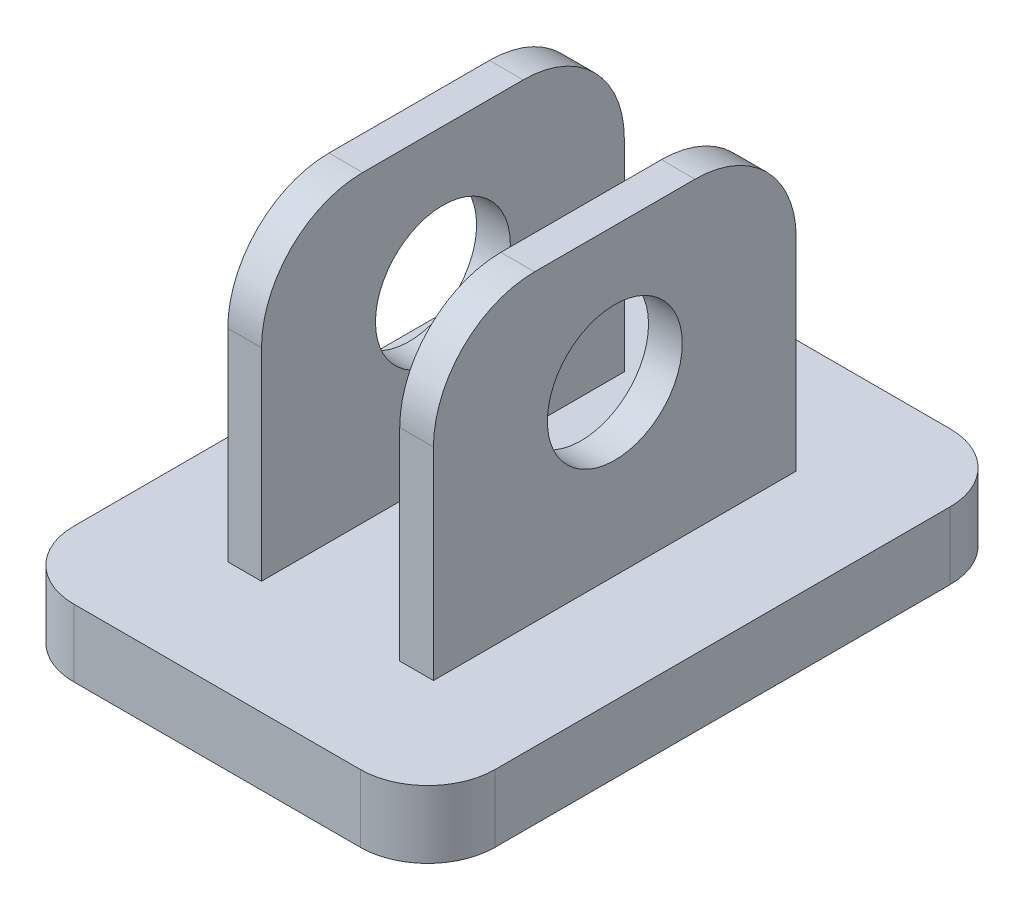
SolidWorks part; units mm, degrees
other "Objet de détail1"
other "Objet de détail2"
other "Dossier de soudure"
other "Cordon de soudure1"
other "Cordon de soudure2"
ref_plane "Plan de face" through (0, 0, 0) normal (0, 0, 1) x (1, 0, 0)
ref_plane "Plan de dessus" through (0, 0, 0) normal (0, 1, 0) x (1, 0, 0)
ref_plane "Plan de droite" through (0, 0, 0) normal (1, 0, 0) x (0, 0, -1)
sketch "Sketch1" plane through (0, 0, 0) normal (0, 1, 0) x (1, 0, 0)
  line L1 (-8.5, -17.5) -> (8.5, -17.5)
  line L2 (-12.5, -13.5) -> (-12.5, 13.5)
  line L3 (-8.5, 17.5) -> (8.5, 17.5)
  line L4 (12.5, -13.5) -> (12.5, 13.5)
  line L5 (0, 17.5) -> (0, -17.5) construction
  line L6 (-12.5, 0) -> (12.5, 0) construction
  arc A0 (8.5, -17.5) -> (12.5, -13.5) centre (8.5, -13.5) ccw
  arc A1 (-8.5, -17.5) -> (-12.5, -13.5) centre (-8.5, -13.5) cw
  arc A2 (8.5, 17.5) -> (12.5, 13.5) centre (8.5, 13.5) cw
  arc A3 (-12.5, 13.5) -> (-8.5, 17.5) centre (-8.5, 13.5) cw
  point P0 (0, 0)
  point P9 (-12.5, -17.5)
  point P12 (12.5, 17.5)
  point P15 (-12.5, 17.5)
  dimension "D3" = 4
  dimension "D1" = 35
  dimension "D2" = 25
extrude "Boss.-Extru.1" add sketch "Sketch1" along normal blind 4
sketch "Sketch2" plane through (0, 4, 0) normal (0, 1, 0) x (1, 0, 0)
  line L0 (0, 17.5) -> (0, -22.848) construction
  line L1 (8.5, 17.5) -> (-8.5, 17.5) construction
  line L2 (-24.7564, 0) -> (26.0286, 0) construction
  line L3 (4.1, 10.7613) -> (-4.1, 10.7613) construction
  line L4 (-4.1, 10.7613) -> (-4.1, -10.7613)
  line L5 (-4.1, 10.7613) -> (-6.1, 10.7613)
  line L6 (-6.1, 10.7613) -> (-6.1, -10.7613)
  line L7 (4.1, -10.7613) -> (-4.1, -10.7613) construction
  line L8 (-4.1, -10.7613) -> (-6.1, -10.7613)
  line L9 (4.1, -10.7613) -> (6.1, -10.7613)
  line L10 (6.1, 10.7613) -> (6.1, -10.7613)
  line L11 (4.1, 10.7613) -> (6.1, 10.7613)
  line L12 (4.1, 10.7613) -> (4.1, -10.7613)
  point P12 (-4.1, 0)
  point P15 (-6.1, 0)
  point P16 (0, -10.7613)
  point P17 (0, 10.7613)
  point P19 (6.1, 0)
  point P20 (4.1, 0)
  dimension "D1" = 4.1
  dimension "D2" = 2
extrude "Boss.-Extru.2" add sketch "Sketch2" along normal blind 18
fillet "Fillet1" radius 6 4 edges at (-5.1, 22, -10.7613) (5.1, 22, -10.7613) (5.1, 22, 10.7613) (-5.1, 22, 10.7613)
sketch "Sketch3" plane through (6.1, 0, 0) normal (1, 0, 0) x (0, 0, -1)
  line L0 (0, 19.9829) -> (0, 7.8956) construction
  circle A0 centre (0, 13.9393) radius 4
  dimension "D1" = 8
extrude "Cut-Extrude1" cut sketch "Sketch3" against normal through all
sketch "Sketch4" plane through (0, 0, 0) normal (0, -1, 0) x (1, 0, 0)
  line L4 (8.5, 17.5) -> (-8.5, 17.5)
  line L5 (-12.5, 13.5) -> (-12.5, -13.5)
  line L6 (-8.5, -17.5) -> (8.5, -17.5)
  line L7 (12.5, -13.5) -> (12.5, 13.5)
  line L8 (8.5, 17.5) -> (-8.5, 17.5)
  line L9 (-12.5, 13.5) -> (-12.5, -13.5)
  line L10 (-8.5, -17.5) -> (8.5, -17.5)
  line L11 (12.5, -13.5) -> (12.5, 13.5)
  arc A4 (12.5, 13.5) -> (8.5, 17.5) centre (8.5, 13.5) ccw
  arc A5 (-8.5, 17.5) -> (-12.5, 13.5) centre (-8.5, 13.5) ccw
  arc A6 (-12.5, -13.5) -> (-8.5, -17.5) centre (-8.5, -13.5) ccw
  arc A7 (8.5, -17.5) -> (12.5, -13.5) centre (8.5, -13.5) ccw
  arc A8 (12.5, 13.5) -> (8.5, 17.5) centre (8.5, 13.5) ccw
  arc A9 (-8.5, 17.5) -> (-12.5, 13.5) centre (-8.5, 13.5) ccw
  arc A10 (-12.5, -13.5) -> (-8.5, -17.5) centre (-8.5, -13.5) ccw
  arc A11 (8.5, -17.5) -> (12.5, -13.5) centre (8.5, -13.5) ccw
  dimension "D1" = 0
